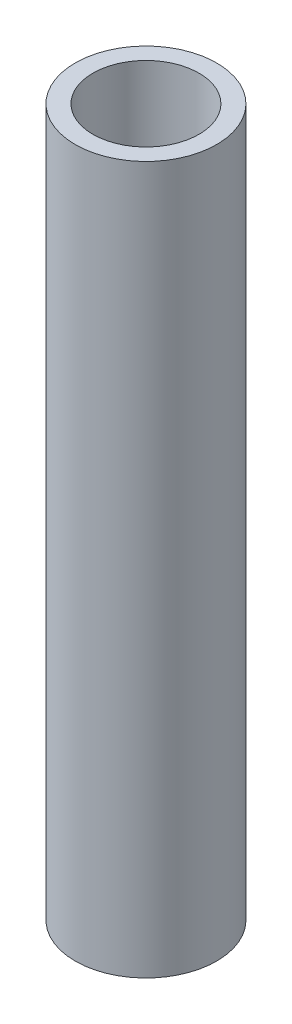
from build123d import *

# Parameters (mm, degrees)
SKETCH1_R           = 4
SKETCH1_R_2         = 3
BOSS_EXTRUDE1_DEPTH = 40


with BuildPart() as part:
    # Sketch1 → Boss-Extrude1 (new body)
    with BuildSketch(Plane(origin=(0, 0, 0), x_dir=(1, 0, 0), z_dir=(0, 1, 0))):
        with Locations(Location((0, 0, 0), (0, 0, 270))):
            Circle(SKETCH1_R)
        with Locations(Location((0, 0, 0), (0, 0, 270))):
            Circle(SKETCH1_R_2, mode=Mode.SUBTRACT)
    extrude(amount=BOSS_EXTRUDE1_DEPTH)


solid = part.part
